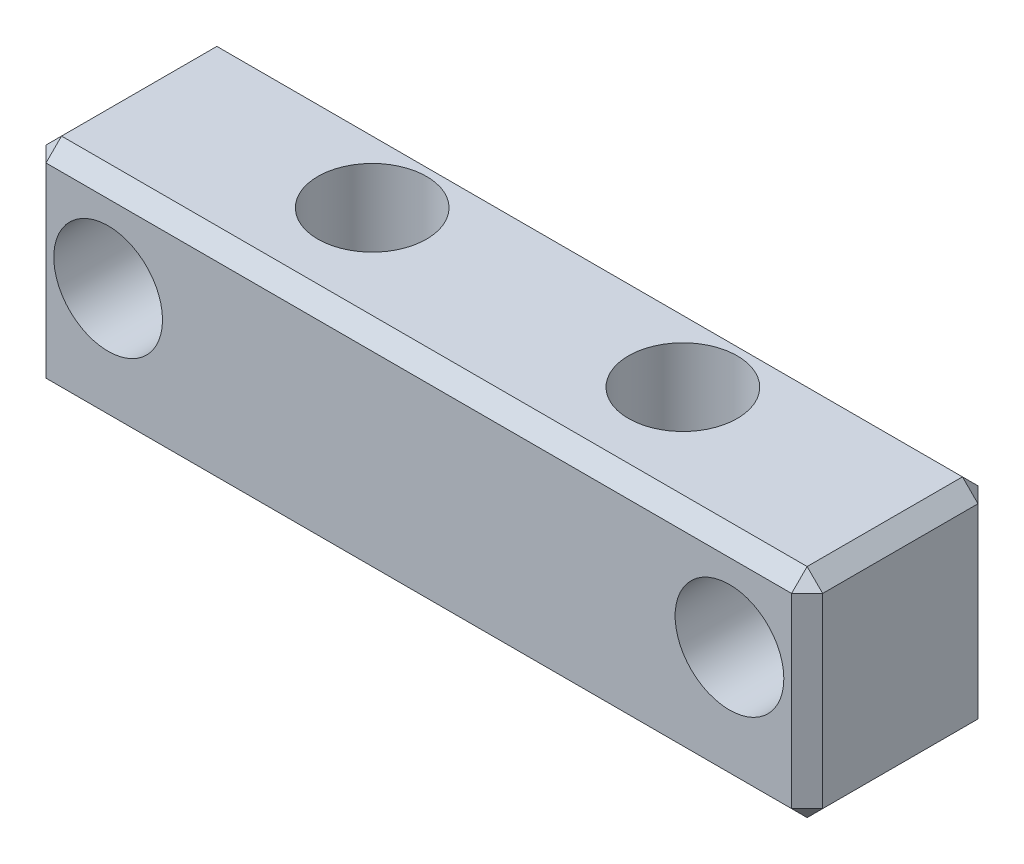
SolidWorks part; units mm, degrees
material "A6061"
ref_plane "Front Plane" through (0, 0, 0) normal (0, 0, 1) x (1, 0, 0)
ref_plane "Top Plane" through (0, 0, 0) normal (0, 1, 0) x (1, 0, 0)
ref_plane "Right Plane" through (0, 0, 0) normal (1, 0, 0) x (0, 0, -1)
sketch "Sketch1" plane through (0, 0, 0) normal (0, 0, 1) x (1, 0, 0)
  line L1 (-12.5, -3.5) -> (12.5, -3.5)
  line L2 (-12.5, -3.5) -> (-12.5, 3.5)
  line L3 (-12.5, 3.5) -> (12.5, 3.5)
  line L4 (12.5, -3.5) -> (12.5, 3.5)
  line L5 (-12.5, -3.5) -> (12.5, 3.5) construction
  line L6 (-12.5, 3.5) -> (12.5, -3.5) construction
  point P0 (0, 0)
  dimension "D1" = 25
  dimension "D2" = 7
extrude "Boss-Extrude1" add sketch "Sketch1" along normal blind 6
hole_wizard "Ø3.5 (3.5) Diameter Hole2" positions "Sketch7" profile "Sketch5" hole size "Ø3.5" standard "GB" end condition through all
sketch "Sketch7" plane through (0, 0, 6) normal (0, 0, 1) x (1, 0, 0)
  line L0 (-10, 0.5) -> (10, 0.5)
  line L3 (12.5, 3.5) -> (-12.5, 3.5) construction
  line L4 (12.5, -3.5) -> (12.5, 3.5) construction
  line L5 (-12.5, 3.5) -> (-12.5, -3.5) construction
  point P0 (-10, 0.5)
  point P2 (10, 0.5)
  dimension "D1" = 3
  dimension "D2" = 2.5
  dimension "D3" = 2.5
sketch "Sketch5" plane through (-10, 0.5, 6) normal (1, 0, 0) x (0, -1, 0)
  line L0 (0, 0) -> (0, 6)
  line L1 (0, 6) -> (1.75, 6)
  line L2 (1.75, 6) -> (1.75, 0)
  line L5 (1.75, 0) -> (0, 0)
  line L11 (0, -6.35) -> (0, 107.95) construction
  dimension "通孔孔直径" = 3.5
  dimension "通孔孔深度" = 6
hole_wizard "Ø3.5 (3.5) Diameter Hole3" positions "Sketch9" profile "Sketch10" hole size "Ø3.5" standard "GB"
sketch "Sketch9" plane through (0, 3.5, 0) normal (0, 1, 0) x (1, 0, 0)
  point P0 (5, -2.5)
  point P3 (-5, -2.5)
sketch "Sketch10" plane through (5, 3.5, 2.5) normal (1, 0, 0) x (0, 0, 1)
  line L0 (0, 0) -> (0, 4.0515)
  line L1 (0, 4.0515) -> (1.75, 3)
  line L2 (1.75, 3) -> (1.75, 0)
  line L5 (1.75, 0) -> (0, 0)
  line L10 (0, 4.0515) -> (-1.75, 3) construction
  line L11 (0, -6.35) -> (0, 107.95) construction
  dimension "孔直径" = 3.5
  dimension "孔深度" = 3
  dimension "导头角度" = 118
chamfer "Chamfer1" distance 0.5 angle 45 12 edges at (0, -3.5, 0) (12.5, 0, 0) (-12.5, 0, 0) (0, 3.5, 0) (-12.5, 3.5, 3) (12.5, 3.5, 3) (12.5, -3.5, 3) (-12.5, -3.5, 3) (-12.5, 0, 6) (0, 3.5, 6) (12.5, 0, 6) (0, -3.5, 6)
